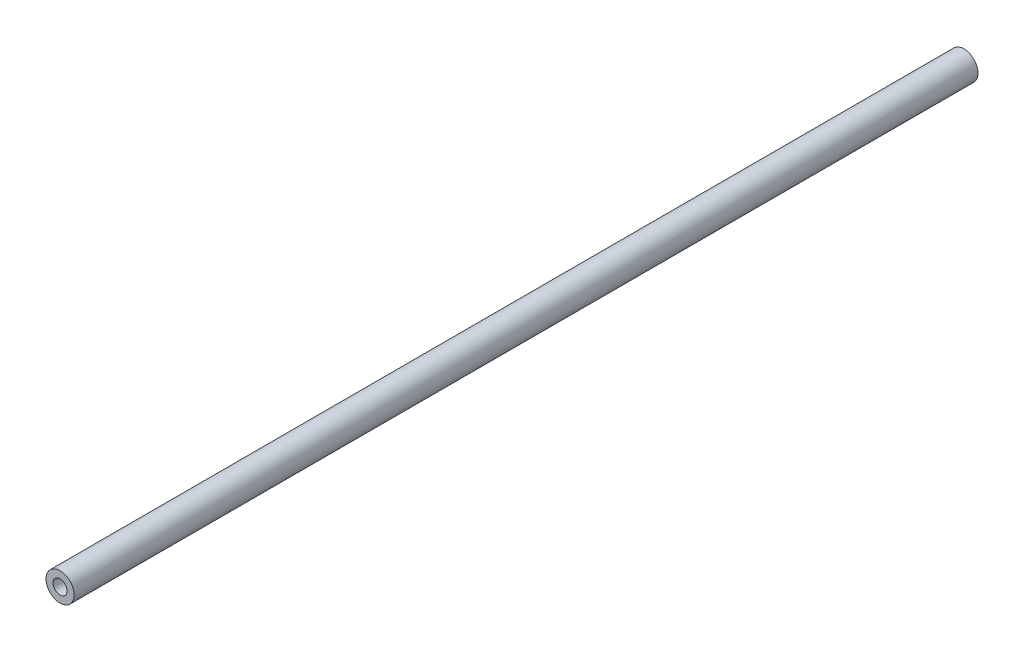
from build123d import *

# Parameters (mm, degrees)
SKETCH1_R             = 5
BOSS_EXTRUDE1_DEPTH   = 321
M6_TAPPED_HOLE1_D     = 5
M6_TAPPED_HOLE1_DEPTH = 15
M6_TAPPED_HOLE1_TIP   = 1.502151548
M6_TAPPED_HOLE2_D     = 5
M6_TAPPED_HOLE2_DEPTH = 15
M6_TAPPED_HOLE2_TIP   = 1.502151548


with BuildPart() as part:
    # Sketch1 → Boss-Extrude1 (new body)
    with BuildSketch(Plane.XY):
        Circle(SKETCH1_R)
    extrude(amount=BOSS_EXTRUDE1_DEPTH)

    # M6 Tapped Hole1
    with Locations(Plane.XY.offset(321)):
        with Locations((0, 0)):
            Hole(M6_TAPPED_HOLE1_D / 2, depth=M6_TAPPED_HOLE1_DEPTH)
            with Locations((0, 0, -(M6_TAPPED_HOLE1_DEPTH + M6_TAPPED_HOLE1_TIP / 2))):  # 118° drill point
                Cone(0, M6_TAPPED_HOLE1_D / 2, M6_TAPPED_HOLE1_TIP, mode=Mode.SUBTRACT)

    # M6 Tapped Hole2
    with Locations(Plane(origin=(0, 0, 0), x_dir=(-1, 0, 0), z_dir=(0, 0, -1))):
        with Locations((0, 0)):
            Hole(M6_TAPPED_HOLE2_D / 2, depth=M6_TAPPED_HOLE2_DEPTH)
            with Locations((0, 0, -(M6_TAPPED_HOLE2_DEPTH + M6_TAPPED_HOLE2_TIP / 2))):  # 118° drill point
                Cone(0, M6_TAPPED_HOLE2_D / 2, M6_TAPPED_HOLE2_TIP, mode=Mode.SUBTRACT)


solid = part.part
